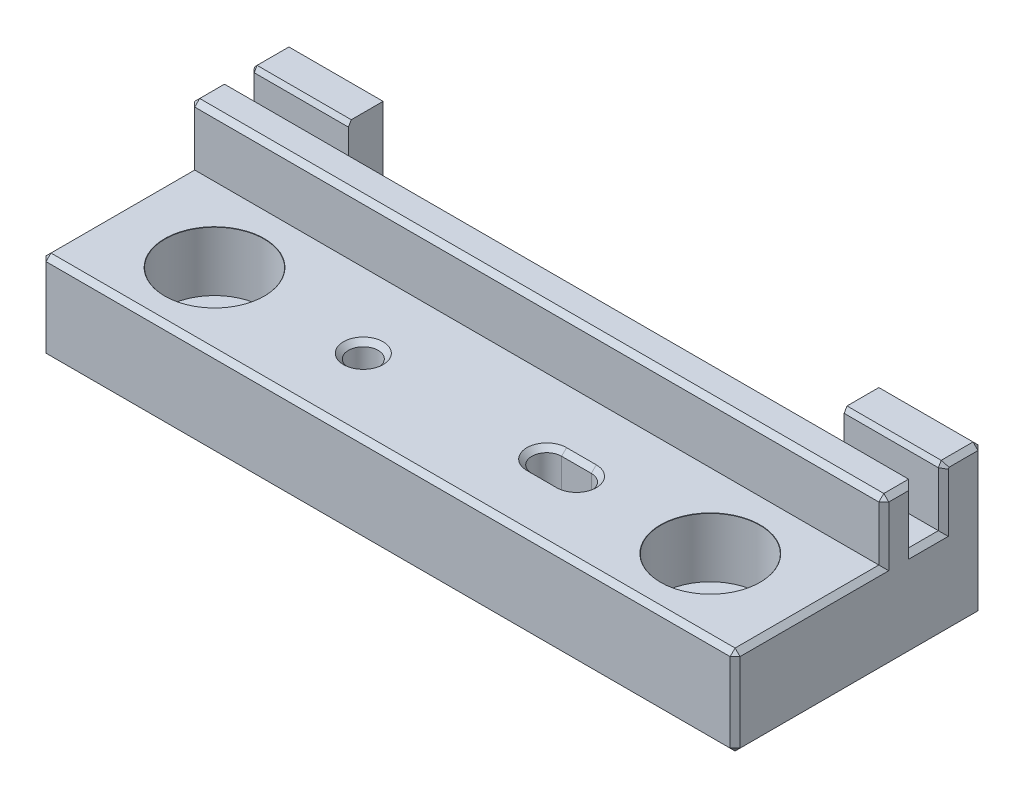
SolidWorks part; units mm, degrees
ref_plane "Front Plane" through (0, 0, 0) normal (0, 0, 1) x (1, 0, 0)
ref_plane "Top Plane" through (0, 0, 0) normal (0, 1, 0) x (1, 0, 0)
ref_plane "Right Plane" through (0, 0, 0) normal (1, 0, 0) x (0, 0, -1)
other "Configuration Table"
sketch "Sketch1" plane through (0, 0, 0) normal (0, 1, 0) x (1, 0, 0)
  line L0 (10, 21) -> (60, 21)
  line L1 (0, 0) -> (70, 0)
  line L2 (0, 0) -> (0, 25)
  line L4 (70, 0) -> (70, 25)
  line L8 (10, 25) -> (10, 21)
  line L12 (60, 25) -> (60, 21)
  line L13 (0, 25) -> (10, 25)
  line L14 (60, 25) -> (70, 25)
  dimension "D1" = 70
  dimension "D2" = 25
  dimension "D3" = 4
  dimension "D4" = 4
  dimension "D5" = 10
  dimension "D6" = 10
extrude "Boss-Extrude1" add sketch "Sketch1" along normal blind 9
sketch "Sketch2" plane through (0, 9, 0) normal (0, 1, 0) x (1, 0, 0)
  line L0 (0, 15) -> (70, 15)
  line L1 (0, 18) -> (70, 18)
  line L2 (0, 18) -> (0, 15)
  line L3 (70, 21) -> (70, 25)
  line L8 (10, 21) -> (0, 21)
  line L9 (60, 21) -> (70, 21)
  line L16 (0, 25) -> (0, 0)
  line L17 (0, 0) -> (70, 0)
  line L18 (70, 0) -> (70, 25)
  line L19 (70, 25) -> (60, 25)
  line L20 (60, 25) -> (60, 21)
  line L21 (60, 21) -> (10, 21)
  line L22 (10, 21) -> (10, 25)
  line L23 (10, 25) -> (0, 25)
  line L24 (0, 25) -> (0, 21)
  line L26 (70, 15) -> (70, 18)
  line L27 (70, 25) -> (60, 25)
  line L28 (60, 25) -> (60, 21)
  line L30 (10, 21) -> (10, 25)
  line L31 (10, 25) -> (0, 25)
  dimension "D2" = 10
  dimension "D1" = 0
  dimension "D3" = 3
extrude "Boss-Extrude2" add sketch "Sketch2" along normal blind 6
sketch "Sketch11" plane through (0, 9, 0) normal (0, 1, 0) x (1, 0, 0)
  line L0 (0, 15) -> (0, 0) construction
  line L1 (70, 0) -> (70, 15) construction
  line L3 (0, 15) -> (70, 15) construction
  point P0 (10, 7.5)
  point P1 (60, 7.5)
  dimension "D1" = 10
  dimension "D2" = 10
  dimension "D4" = 7.5
hole_wizard "CBORE for M5 Slotted cheese head screws1" positions "Sketch11" profile "Sketch12" counterbore size "M5" standard "GB" end condition through all
sketch "Sketch12" plane through (10, 9, -7.5) normal (1, 0, 0) x (0, 0, 1)
  line L0 (0, 0) -> (0, 9)
  line L1 (0, 9) -> (2.75, 9)
  line L3 (2.75, 9) -> (2.75, 6)
  line L4 (5, 6) -> (2.75, 6)
  line L5 (5, 6) -> (5, 0.025)
  line L6 (5, 0.025) -> (5.025, 0)
  line L7 (5.025, 0) -> (0, 0)
  line L8 (-5, 0.025) -> (-5.025, 0) construction
  line L11 (0, -6.35) -> (0, 107.95) construction
  dimension "通孔孔直径" = 5.5
  dimension "通孔孔深度" = 9
  dimension "柱形沉头孔直径" = 10
  dimension "柱形沉头孔深度" = 6
  dimension "近端锥形沉头孔直径" = 10.05
  dimension "近端锥形沉头孔角度" = 90
sketch "Sketch13" plane through (0, 9, 0) normal (0, 1, 0) x (1, 0, 0)
  circle A0 centre (45, 7.5027) radius 1.5
  circle A1 centre (25, 7.5027) radius 1.5
  circle A2 centre (60, 7.5) radius 2.75 construction
  dimension "D4" = 3
  dimension "D5" = 3
  dimension "D1" = 0.0027
  dimension "D2" = 15
  dimension "D3" = 20
extrude "Cut-Extrude1" cut sketch "Sketch13" against normal through all
chamfer "Chamfer3" distance 0.5 angle 30 2 edges at (65, 15, -21) (5, 15, -21)
chamfer "Chamfer9" distance 2 angle 45 1 edges at (35, 9, -21)
fillet "Fillet1" radius 1 2 edges at (60, 3.5, -21) (10, 3.5, -21)
chamfer "Chamfer6" distance 0.5 31 edges at (0, 12, -15) (0, 9, -7.5) (0, 0, -12.5) (10, 7.5, -25) (5, 15, -25) (5, 0, -25) (0, 7.5, -25) (0, 15, -23.1443) (0, 14.75, -21.1443) (0, 11.75, -21) (0, 9, -19.5) (0, 12, -18) (0, 15, -16.5) (65, 15, -25) (60, 7.5, -25) (65, 0, -25) (70, 9, -19.5) (70, 11.75, -21) (70, 14.75, -21.1443) (70, 15, -23.1443) (70, 7.5, -25) (70, 0, -12.5) (0, 4.5, 0) (35, 9, 0) (35, 0, 0) (70, 4.5, 0) (70, 9, -7.5) (70, 12, -15) (70, 12, -18) (70, 15, -16.5) (35, 15, -15)
chamfer "Chamfer7" distance 0.5 2 edges at (25, 9, -6.0027) (25, 0, -6.0027)
sketch "Sketch14" plane through (0, 9, 0) normal (0, 1, 0) x (1, 0, 0)
  line L0 (43.5, 7.5027) -> (46.5, 7.5027) construction
  line L1 (43.5, 9.0027) -> (46.5, 9.0027)
  line L2 (43.5, 6.0027) -> (46.5, 6.0027)
  arc A1 (43.5, 9.0027) -> (43.5, 6.0027) centre (43.5, 7.5027) ccw
  arc A2 (46.5, 6.0027) -> (46.5, 9.0027) centre (46.5, 7.5027) ccw
  circle A3 centre (45, 7.5027) radius 1.5 construction
  point P5 (45, 7.5027)
  dimension "D1" = 3
  dimension "D2" = 0
extrude "Cut-Extrude2" cut sketch "Sketch14" against normal through all
chamfer "Chamfer8" distance 0.5 8 edges at (45, 9, -6.0027) (45, 9, -9.0027) (48, 9, -7.5027) (42, 9, -7.5027) (45, 0, -6.0027) (45, 0, -9.0027) (48, 0, -7.5027) (42, 0, -7.5027)
